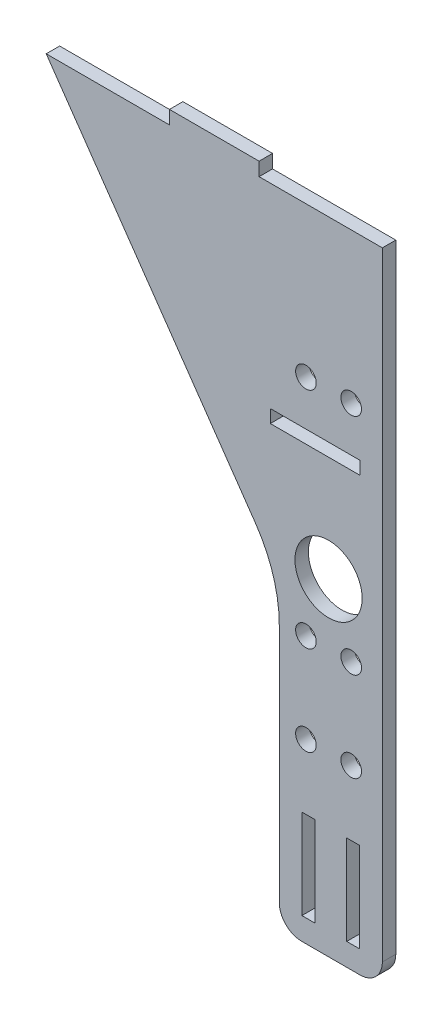
SolidWorks part; units mm, degrees
ref_plane "Front Plane" through (0, 0, 0) normal (0, 0, 1) x (1, 0, 0)
ref_plane "Top Plane" through (0, 0, 0) normal (0, 1, 0) x (1, 0, 0)
ref_plane "Right Plane" through (0, 0, 0) normal (1, 0, 0) x (0, 0, -1)
sketch "Sketch1" plane through (0, 0, 0) normal (0, 0, 1) x (1, 0, 0)
  line L0 (-6.5, 25) -> (-6.5, 5) construction
  line L1 (0, 0) -> (-23, 0)
  line L2 (0, 0) -> (0, 143)
  line L3 (0, 143) -> (-27.5, 143)
  line L4 (-23, 0) -> (-23, 68)
  line L5 (-16.5, 25) -> (-16.5, 5) construction
  line L11 (-17.95, 25) -> (-15.05, 25)
  line L12 (-17.95, 25) -> (-17.95, 5)
  line L13 (-17.95, 5) -> (-15.05, 5)
  line L14 (-15.05, 25) -> (-15.05, 5)
  line L17 (-7.95, 5) -> (-5.05, 5)
  line L18 (-7.95, 5) -> (-7.95, 25)
  line L19 (-7.95, 25) -> (-5.05, 25)
  line L20 (-5.05, 5) -> (-5.05, 25)
  line L25 (-23, 68) -> (-75, 143)
  line L26 (-47.5, 143) -> (-47.5, 146)
  line L27 (-47.5, 146) -> (-27.5, 146)
  line L28 (-27.5, 143) -> (-27.5, 146)
  line L30 (-75, 143) -> (-47.5, 143)
  dimension "D2" = 6.5
  dimension "D3" = 10
  dimension "D4" = 27.5
  dimension "D5" = 23
  dimension "D6" = 47.5
  dimension "D7" = 5
  dimension "D8" = 146
  dimension "D9" = 68
  dimension "D10" = 143
  dimension "D11" = 2.9
extrude "Boss-Extrude1" add sketch "Sketch1" along normal blind 3
fillet "Fillet1" radius 5 2 edges at (0, 0, 1.5) (-23, 0, 1.5)
fillet "Fillet2" radius 30 1 edges at (-23, 68, 1.5)
sketch "Sketch3" plane through (0, 0, 0) normal (0, 0, -1) x (-1, 0, 0)
  line L0 (0, 5) -> (0, 143) construction
  line L1 (6.95, 109.5) -> (17.05, 109.5) construction
  line L2 (6.95, 109.5) -> (6.95, 59.5) construction
  line L3 (6.95, 59.5) -> (17.05, 59.5) construction
  line L4 (17.05, 109.5) -> (17.05, 59.5) construction
  line L5 (0, 143) -> (27.5, 143) construction
  circle A0 centre (12, 73) radius 7.5
  circle A1 centre (17.05, 59.5) radius 2.3
  circle A2 centre (6.95, 59.5) radius 2.3
  circle A3 centre (17.05, 109.5) radius 2.3
  circle A4 centre (6.95, 109.5) radius 2.3
  dimension "D1" = 4.6
  dimension "D2" = 13.5
  dimension "D6" = 15
  dimension "D7" = 12
  dimension "D8" = 70
  dimension "D3" = 10.1
  dimension "D4" = 50
  dimension "D5" = 5.05
extrude "Cut-Extrude1" cut sketch "Sketch3" against normal up to next
sketch "Sketch5" plane through (0, 0, 0) normal (0, 0, -1) x (-1, 0, 0)
  line L0 (25, 96.55) -> (25, 99.45) construction
  line L1 (25, 99.45) -> (5, 99.45) construction
  line L2 (5, 96.55) -> (25, 96.55) construction
  line L3 (5, 99.45) -> (5, 96.55) construction
  line L4 (25, 96.55) -> (25, 99.45)
  line L5 (25, 99.45) -> (5, 99.45)
  line L6 (5, 96.55) -> (25, 96.55)
  line L7 (5, 99.45) -> (5, 96.55)
extrude "Cut-Extrude2" cut sketch "Sketch5" against normal blind 3
sketch "Sketch6" plane through (0, 0, 3) normal (0, 0, 1) x (1, 0, 0)
  line L0 (-17.05, 59.5) -> (-17.05, 39.5) construction
  line L1 (0, 5) -> (0, 143) construction
  line L2 (-18, 0) -> (-5, 0) construction
  circle A0 centre (-17.05, 39.5) radius 2.3
  circle A1 centre (-6.95, 39.5) radius 2.3
  dimension "D1" = 4.6
  dimension "D2" = 4.6
  dimension "D3" = 10.1
  dimension "D4" = 6.95
  dimension "D5" = 39.5
extrude "Cut-Extrude3" cut sketch "Sketch6" against normal blind 3
